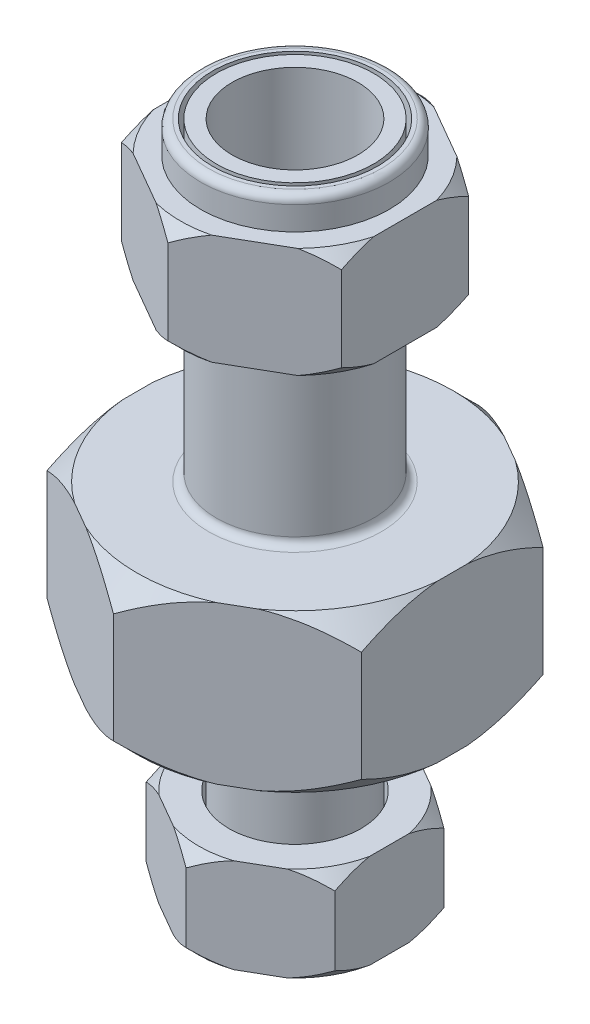
from build123d import *

# Parameters (mm, degrees)
BOSS_EXTRUDE1_DEPTH = 10
SKETCH2_R           = 5
BOSS_EXTRUDE2_DEPTH = 20
SKETCH3_R           = 4
BOSS_EXTRUDE3_DEPTH = 14
SKETCH4_R           = 3
CUT_EXTRUDE1_DEPTH  = 30
SKETCH5_R           = 4
CUT_EXTRUDE2_DEPTH  = 17
SKETCH6_R           = 6
SKETCH6_R_2         = 5.25
BOSS_EXTRUDE4_DEPTH = 2
SKETCH7_R           = 5.25
BOSS_EXTRUDE5_DEPTH = 7
SKETCH11_R          = 4.75
SKETCH11_R_2        = 4.2
BOSS_EXTRUDE6_DEPTH = 1
SKETCH12_R          = 4.2
BOSS_EXTRUDE7_DEPTH = 6
FILLET1_R           = 0.5
FILLET2_R           = 0.5
FILLET3_R           = 0.5


with BuildPart() as part:
    # Sketch1 → Boss-Extrude1 (new body)
    with BuildSketch(Plane(origin=(0, 0, 0), x_dir=(1, 0, 0), z_dir=(0, 1, 0))):
        Polygon((0, -11.547005384), (10, -5.773502692), (10, 5.773502692), (0, 11.547005384), (-10, 5.773502692), (-10, -5.773502692), align=None)
    extrude(amount=BOSS_EXTRUDE1_DEPTH)

    # Sketch2 → Boss-Extrude2 (add)
    with BuildSketch(Plane(origin=(0, 10, 0), x_dir=(1, 0, 0), z_dir=(0, 1, 0))):
        with Locations(Location((0, 0, 0), (0, 0, 270))):
            Circle(SKETCH2_R)
    extrude(amount=BOSS_EXTRUDE2_DEPTH)

    # Sketch3 → Boss-Extrude3 (add)
    with BuildSketch(Plane.XZ):
        with Locations(Location((0, 0, 0), (0, 0, 270))):
            Circle(SKETCH3_R)
    extrude(amount=BOSS_EXTRUDE3_DEPTH)

    # Sketch4 → Cut-Extrude1 (cut)
    with BuildSketch(Plane.XZ.offset(14)):
        with Locations(Location((0, 0, 0), (0, 0, 270))):
            Circle(SKETCH4_R)
    extrude(amount=-CUT_EXTRUDE1_DEPTH, mode=Mode.SUBTRACT)

    # Sketch5 → Cut-Extrude2 (cut)
    with BuildSketch(Plane(origin=(0, 30, 0), x_dir=(1, 0, 0), z_dir=(0, 1, 0))):
        with Locations(Location((0, 0, 0), (0, 0, 90))):
            Circle(SKETCH5_R)
    extrude(amount=-CUT_EXTRUDE2_DEPTH, mode=Mode.SUBTRACT)


with BuildPart() as body_2:
    # Sketch6 → Boss-Extrude4 (new body)
    with BuildSketch(Plane(origin=(0, 30, 0), x_dir=(1, 0, 0), z_dir=(0, 1, 0))):
        with Locations(Location((0, 0, 0), (0, 0, 270))):
            Circle(SKETCH6_R)
        with Locations(Location((0, 0, 0), (0, 0, 270))):
            Circle(SKETCH6_R_2, mode=Mode.SUBTRACT)
    extrude(amount=-BOSS_EXTRUDE4_DEPTH)

    # Sketch7 → Boss-Extrude5 (add)
    with BuildSketch(Plane.XZ.offset(-28)):
        Polygon((0, 8.082903769), (-7, 4.041451884), (-7, -4.041451884), (0, -8.082903769), (7, -4.041451884), (7, 4.041451884), align=None)
        with Locations(Location((0, 0, 0), (0, 0, 90))):
            Circle(SKETCH7_R, mode=Mode.SUBTRACT)
    extrude(amount=BOSS_EXTRUDE5_DEPTH)


with BuildPart() as body_3:
    # Sketch11 → Boss-Extrude6 (new body)
    with BuildSketch(Plane.XZ.offset(14)):
        with Locations(Location((0, 0, 0), (0, 0, 270))):
            Circle(SKETCH11_R)
        with Locations(Location((0, 0, 0), (0, 0, 270))):
            Circle(SKETCH11_R_2, mode=Mode.SUBTRACT)
    extrude(amount=-BOSS_EXTRUDE6_DEPTH)

    # Sketch12 → Boss-Extrude7 (add)
    with BuildSketch(Plane(origin=(0, -13, 0), x_dir=(1, 0, 0), z_dir=(0, 1, 0))):
        Polygon((0, 6.92820323), (-6, 3.464101615), (-6, -3.464101615), (0, -6.92820323), (6, -3.464101615), (6, 3.464101615), align=None)
        with Locations(Location((0, 0, 0), (0, 0, 90))):
            Circle(SKETCH12_R, mode=Mode.SUBTRACT)
    extrude(amount=BOSS_EXTRUDE7_DEPTH)


with BuildPart() as cut_revolve2_tool:
    # Sketch9 → Cut-Revolve2 (revolve)
    with BuildSketch(Plane(origin=(0, 0, 0), x_dir=(0, 0, -1), z_dir=(1, 0, 0))):
        Polygon((-7.282903769, 28), (-8.082903769, 27.2), (-8.082903769, 28), align=None)
        Polygon((-8.082903769, 21), (-7.282903769, 21), (-8.082903769, 21.8), align=None)
        Polygon((-11.547005384, 10), (-11.547005384, 8.5), (-10.047005384, 10), align=None)
        Polygon((-10.047005384, 0), (-11.547005384, 0), (-11.547005384, 1.5), align=None)
        Polygon((-6.92820323, -7), (-6.92820323, -7.8), (-6.12820323, -7), align=None)
        Polygon((-6.12820323, -13), (-6.92820323, -13), (-6.92820323, -12.2), align=None)
    revolve(axis=Axis((0, 30, 0), (0, 1, 0)))


with BuildPart() as part_1:
    add(part.part)

    # Cut-Revolve2: cut by cut_revolve2_tool
    add(cut_revolve2_tool.part, mode=Mode.SUBTRACT)

    # Fillet2
    fillet2_edges = [part_1.edges().sort_by_distance(p)[0] for p in [
        (0, 10, -5),
        (0, 0, 4),
    ]]
    fillet(fillet2_edges, radius=FILLET2_R)


with BuildPart() as body_2_1:
    add(body_2.part)

    # Cut-Revolve2: cut by cut_revolve2_tool
    add(cut_revolve2_tool.part, mode=Mode.SUBTRACT)

    # Fillet1
    fillet1_edges = [body_2_1.edges().sort_by_distance(p)[0] for p in [
        (0, 30, -6),
    ]]
    fillet(fillet1_edges, radius=FILLET1_R)


with BuildPart() as body_3_1:
    add(body_3.part)

    # Cut-Revolve2: cut by cut_revolve2_tool
    add(cut_revolve2_tool.part, mode=Mode.SUBTRACT)

    # Fillet3
    fillet3_edges = [body_3_1.edges().sort_by_distance(p)[0] for p in [
        (0, -14, 4.75),
    ]]
    fillet(fillet3_edges, radius=FILLET3_R)


solid = Compound([part_1.part, body_2_1.part, body_3_1.part])
